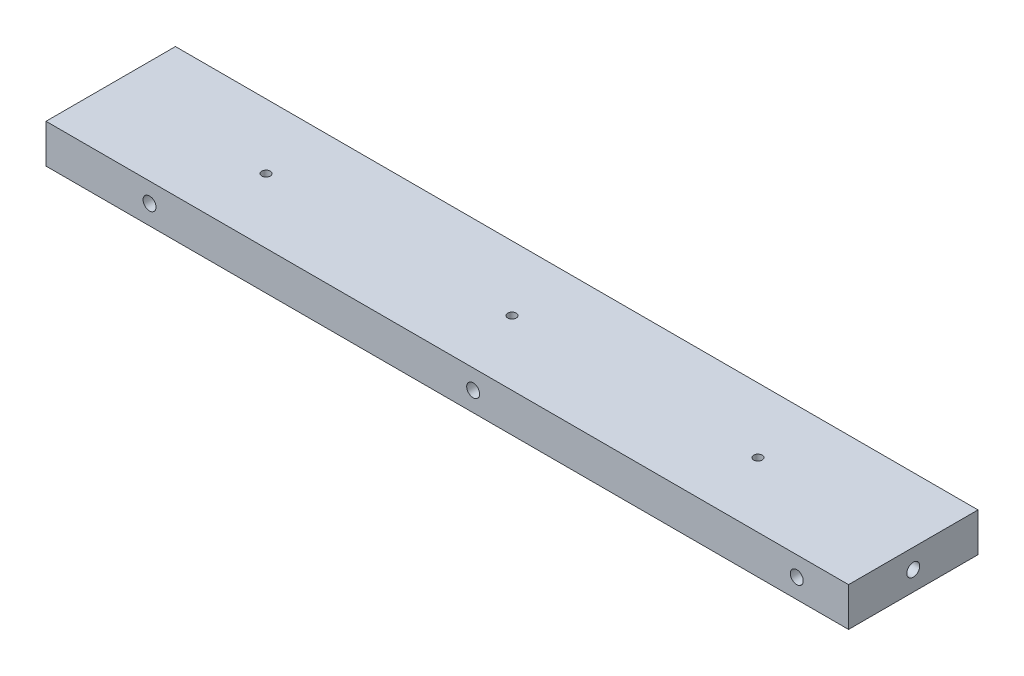
from build123d import *

# Parameters (mm, degrees)
SKETCH_1_W             = 310
SKETCH_1_H             = 50
EXTRUDE_1_DEPTH        = 7.5
HOLE_WIZARD_M6_1_D     = 5
HOLE_WIZARD_M6_1_DEPTH = 17
HOLE_WIZARD_M6_1_TIP   = 1.502151548
HOLE_WIZARD_M6_2_D     = 5
HOLE_WIZARD_M6_2_DEPTH = 17
HOLE_WIZARD_M6_2_TIP   = 1.502151548
HOLE_WIZARD_M6_3_D     = 5
HOLE_WIZARD_M6_3_DEPTH = 17
HOLE_WIZARD_M6_3_TIP   = 1.502151548
HOLE_WIZARD_M4_1_D     = 3.3


with BuildPart() as part:
    # 草图1 → 凸台-拉伸1 (new, symmetric)
    with BuildSketch(Plane(origin=(0, 0, 0), x_dir=(1, 0, 0), z_dir=(0, 1, 0))):
        Rectangle(SKETCH_1_W, SKETCH_1_H)
    extrude(amount=EXTRUDE_1_DEPTH, both=True)

    # M6 螺纹孔1
    with Locations(Plane.XY.offset(25)):
        with Locations((-115, 0), (10, 0), (135, 0)):
            Hole(HOLE_WIZARD_M6_1_D / 2, depth=HOLE_WIZARD_M6_1_DEPTH)
            with Locations((0, 0, -(HOLE_WIZARD_M6_1_DEPTH + HOLE_WIZARD_M6_1_TIP / 2))):  # 118° drill point
                Cone(0, HOLE_WIZARD_M6_1_D / 2, HOLE_WIZARD_M6_1_TIP, mode=Mode.SUBTRACT)

    # M6 螺纹孔2
    with Locations(Plane(origin=(155, 0, 0), x_dir=(0, 0, -1), z_dir=(1, 0, 0))):
        with Locations((0, 0)):
            Hole(HOLE_WIZARD_M6_2_D / 2, depth=HOLE_WIZARD_M6_2_DEPTH)
            with Locations((0, 0, -(HOLE_WIZARD_M6_2_DEPTH + HOLE_WIZARD_M6_2_TIP / 2))):  # 118° drill point
                Cone(0, HOLE_WIZARD_M6_2_D / 2, HOLE_WIZARD_M6_2_TIP, mode=Mode.SUBTRACT)

    # M6 螺纹孔3
    with Locations(Plane.ZY.offset(155)):
        with Locations((0, 0)):
            Hole(HOLE_WIZARD_M6_3_D / 2, depth=HOLE_WIZARD_M6_3_DEPTH)
            with Locations((0, 0, -(HOLE_WIZARD_M6_3_DEPTH + HOLE_WIZARD_M6_3_TIP / 2))):  # 118° drill point
                Cone(0, HOLE_WIZARD_M6_3_D / 2, HOLE_WIZARD_M6_3_TIP, mode=Mode.SUBTRACT)

    # M4 螺纹孔1 (through all)
    with Locations(Plane(origin=(0, 7.5, 0), x_dir=(1, 0, 0), z_dir=(0, 1, 0))):
        with Locations((-95, 0), (0, 0), (95, 0)):
            Hole(HOLE_WIZARD_M4_1_D / 2)


solid = part.part
